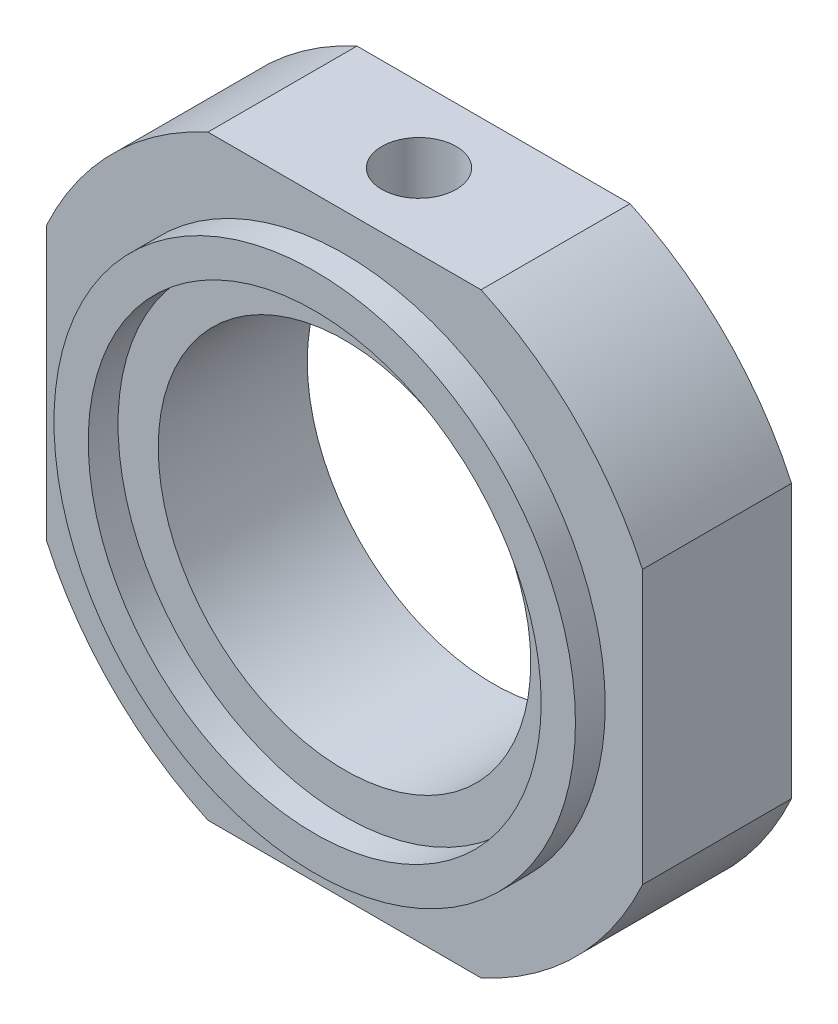
SolidWorks part; units mm, degrees
ref_plane "Front Plane" through (0, 0, 0) normal (0, 0, 1) x (1, 0, 0)
ref_plane "Top Plane" through (0, 0, 0) normal (0, 1, 0) x (1, 0, 0)
ref_plane "Right Plane" through (0, 0, 0) normal (1, 0, 0) x (0, 0, -1)
sketch "Sketch7" plane through (0, 0, 0) normal (0, 0, 1) x (1, 0, 0)
  circle A0 centre (0, 0) radius 11
  dimension "D1" = 22
extrude "Boss-Extrude1" add sketch "Sketch7" along normal mid plane 5
sketch "Sketch8" plane through (0, 0, 2.5) normal (0, 0, 1) x (1, 0, 0)
  circle A0 centre (0, 0) radius 7.6
  circle A1 centre (0, 0) radius 8.75
  dimension "D1" = 15.2
  dimension "D2" = 17.5
extrude "Boss-Extrude2" add sketch "Sketch8" along normal blind 1
hole_wizard "M14x1.5 Tapped Hole1" positions "Sketch10" profile "Sketch9" tap size "M14x1.5" standard "Gb" end condition through all
sketch "Sketch10" plane through (0, 0, -2.5) normal (0, 0, -1) x (-1, 0, 0)
  point P0 (0, 0)
sketch "Sketch9" plane through (0, 0, -2.5) normal (1, 0, 0) x (0, 1, 0)
  line L0 (0, 0) -> (0, 6)
  line L1 (0, 6) -> (6.25, 6)
  line L2 (6.25, 6) -> (6.25, 0)
  line L5 (6.25, 0) -> (0, 0)
  line L11 (0, -6.35) -> (0, 107.95) construction
  dimension "通孔螺纹孔钻头直径" = 12.5
  dimension "通孔螺纹孔钻头深度" = 6
cosmetic thread "Hole Thread3" parameters "D2"=14
sketch "Sketch13" plane through (0, 0, -2.5) normal (0, 0, -1) x (-1, 0, 0)
  line L1 (-10, 10) -> (10, 10)
  line L2 (-10, 10) -> (-10, -10)
  line L3 (-10, -10) -> (10, -10)
  line L4 (10, 10) -> (10, -10)
  line L5 (-10, 10) -> (10, -10) construction
  line L6 (-10, -10) -> (10, 10) construction
  point P0 (0, 0)
  dimension "D1" = 20
  dimension "D2" = 20
extrude "Cut-Extrude1" cut sketch "Sketch13" against normal through all flip side to cut
hole_wizard "M3 Tapped Hole3" positions "Sketch15" profile "Sketch14" tap size "M3" standard "Gb"
sketch "Sketch15" plane through (0, 10, 0) normal (0, 1, 0) x (1, 0, 0)
  point P0 (0, 0)
sketch "Sketch14" plane through (0, 10, 0) normal (1, 0, 0) x (0, 0, 1)
  line L0 (0, 0) -> (0, 3.75)
  line L1 (0, 3.75) -> (1.25, 3.75)
  line L2 (1.25, 3.75) -> (1.25, 0)
  line L5 (1.25, 0) -> (0, 0)
  line L11 (0, -6.35) -> (0, 107.95) construction
  dimension "通孔螺纹孔钻头直径" = 2.5
  dimension "通孔螺纹孔钻头深度" = 3.75
cosmetic thread "Hole Thread5" parameters "D2"=3
